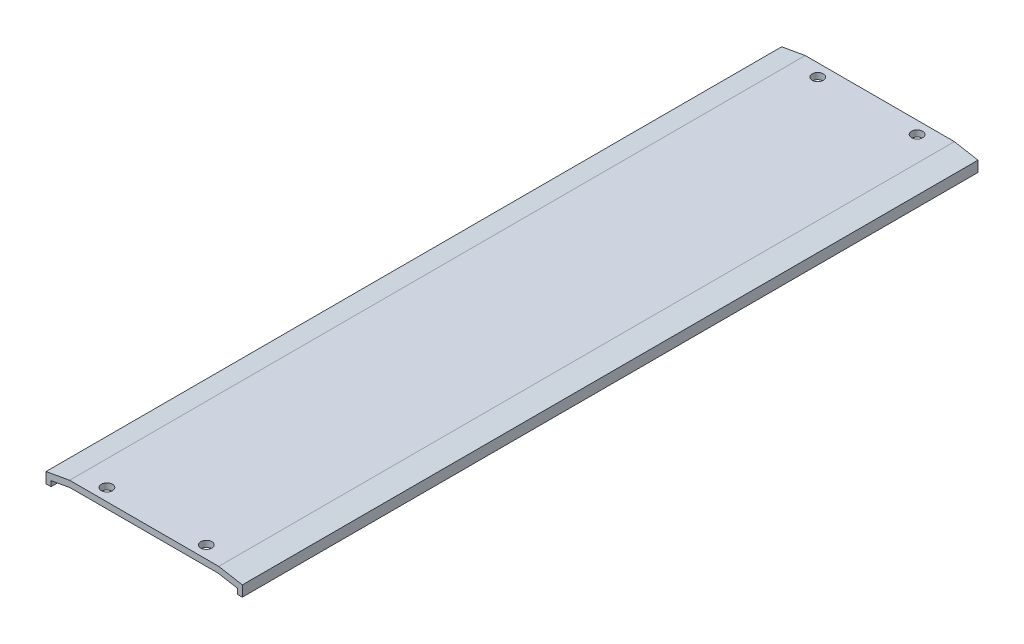
SolidWorks part; units mm, degrees
material "GY-D-79MG 型材"
ref_plane "前视基准面" through (0, 0, 0) normal (0, 0, 1) x (1, 0, 0)
ref_plane "上视基准面" through (0, 0, 0) normal (0, 1, 0) x (1, 0, 0)
ref_plane "右视基准面" through (0, 0, 0) normal (1, 0, 0) x (0, 0, -1)
sketch "草图1" plane through (0, 0, 0) normal (0, 0, 1) x (1, 0, 0)
  line L0 (0, 0) -> (0, 49.2018) construction
  line L1 (-37.5, 0) -> (-39.5, 0)
  line L2 (-39.5, 0) -> (-39.5, 4.3)
  line L3 (-39.5, 4.3) -> (-30, 6)
  line L4 (-30, 6) -> (30, 6)
  line L5 (-37.5, 0) -> (-37.5, 2.1221)
  line L6 (-37.5, 2.1221) -> (-29.8, 3.5)
  line L7 (-29.8, 3.5) -> (29.8, 3.5)
  line L8 (37.5, 2.1221) -> (29.8, 3.5)
  line L9 (37.5, 0) -> (37.5, 2.1221)
  line L10 (39.5, 4.3) -> (30, 6)
  line L11 (39.5, 0) -> (39.5, 4.3)
  line L12 (37.5, 0) -> (39.5, 0)
  point P12 (0, 3.5)
  point P15 (0, 6)
  dimension "D1" = 79
  dimension "D2" = 75
  dimension "D3" = 2.5
  dimension "D4" = 4.3
  dimension "D5" = 6
  dimension "D6" = 59.6
  dimension "D7" = 60
extrude "凸台-拉伸1" add sketch "草图1" along normal mid plane 296
sketch "草图2" plane through (0, 6, 0) normal (0, 1, 0) x (1, 0, 0)
  line L0 (30, -148) -> (-30, -148) construction
  line L1 (0, -148) -> (0, -116.2041) construction
  circle A0 centre (-20, -143) radius 2.25
  circle A1 centre (20, -143) radius 2.25
  dimension "D1" = 4.5
  dimension "D2" = 4.5
  dimension "D4" = 5
  dimension "D3" = 40
extrude "切除-拉伸1" cut sketch "草图2" against normal blind 10
mirror "镜向1" about plane through (0, 0, 0) normal (0, 0, 1) of "切除-拉伸1"
